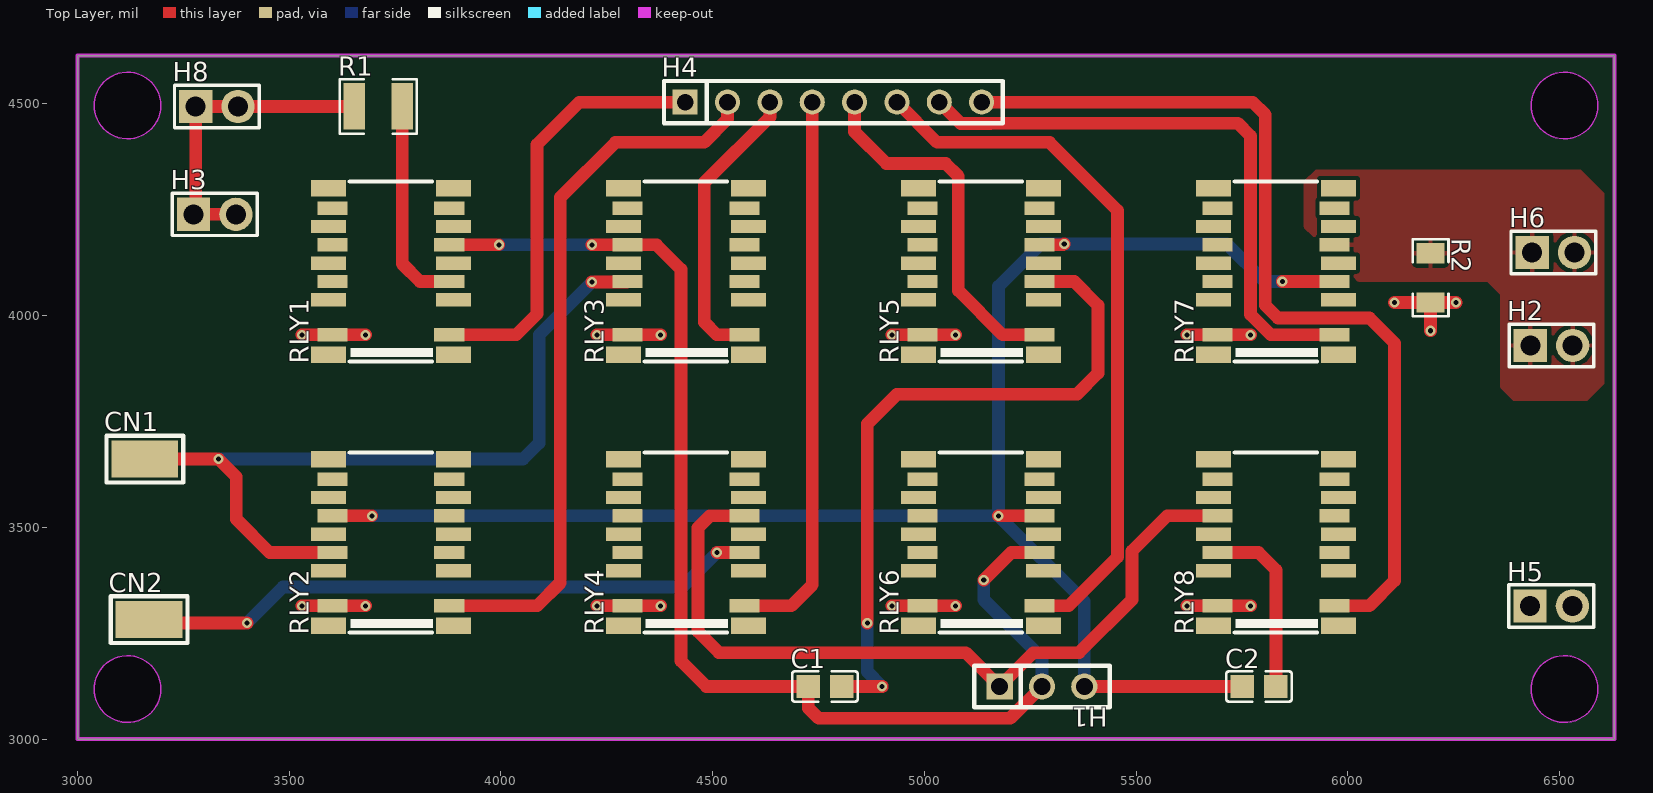
[diagram p0: Top Layer view]
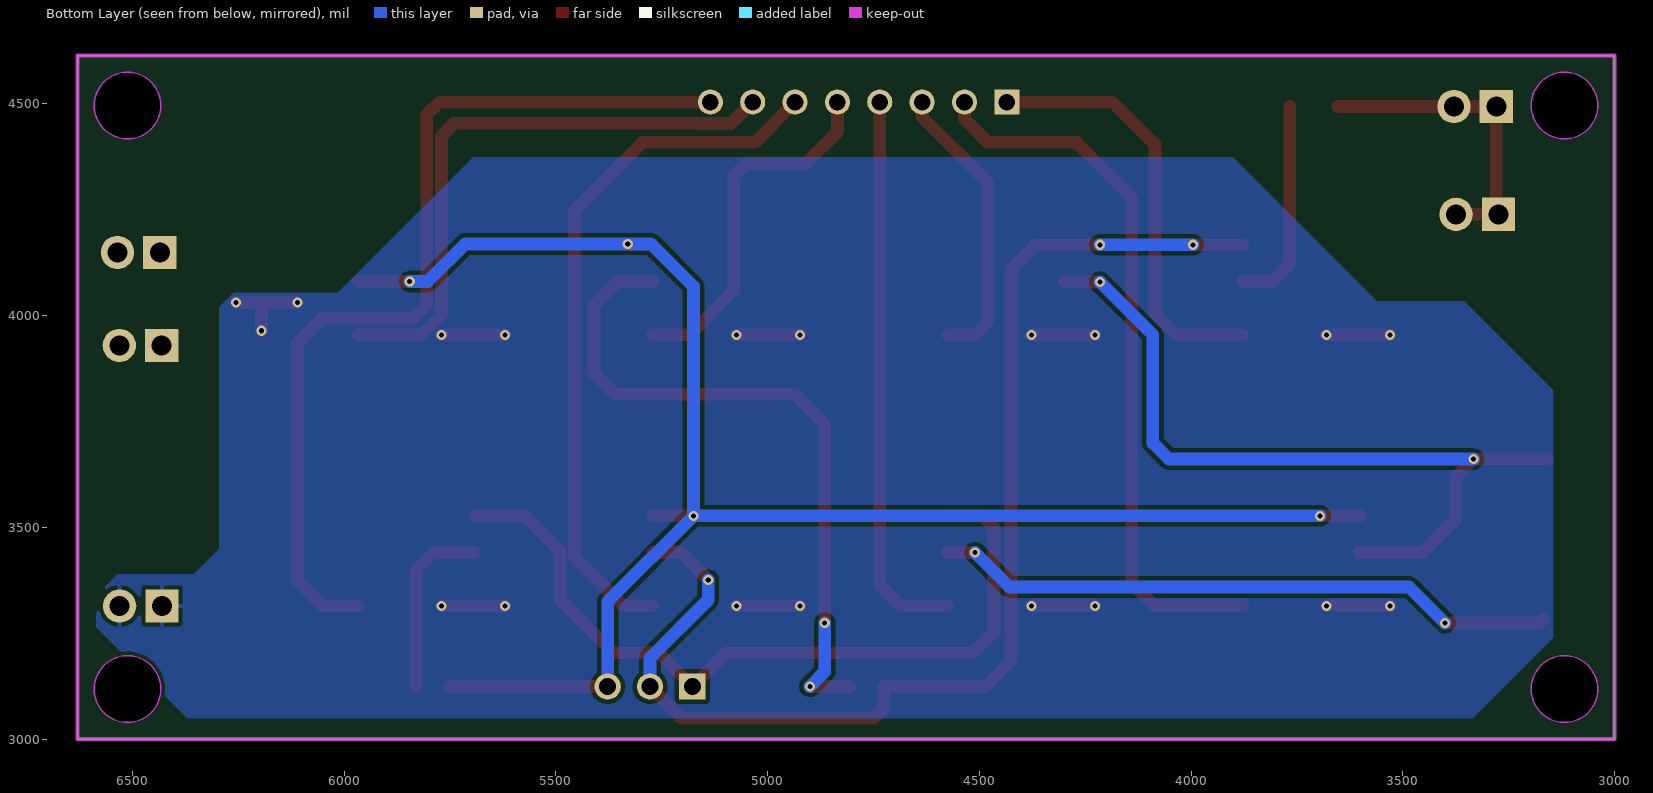
[diagram p1: Bottom Layer view, seen from below]
# Altium PCB MISC51843.pcbdoc
Units mil, origin at the board's own origin, x right, y up, seen from the top; angles counter-clockwise.
Board outline 3629.38 x 1614.17 mil, 2 copper layers (Top Layer, Bottom Layer), stack 62.206 mil thick; 21 components, 19 nets, 175 pads, 32 vias.

## Layer stack, top to bottom
Top Solder Mask Layer: solder mask 0.394, Dk 3.3
Top Layer: signal copper 1.379
Dielectric1: surface 59.449, FR4, Dk 4.5
Bottom Layer: signal copper 1.378
Bottom Solder Mask Layer: solder mask 0.394, Dk 3.3

## Board outline
3000,4614.17 3000,3000 6629.38,3000 6629.38,4614.17
cut-out: 3196.85,4496.06 cw(c3118.11,4496.06) 3039.37,4496.06 cw(c3118.11,4496.06)
cut-out: 6590.01,4496.06 cw(c6511.27,4496.06) 6432.53,4496.06 cw(c6511.27,4496.06)
cut-out: 6590.01,3118.11 cw(c6511.27,3118.11) 6432.53,3118.11 cw(c6511.27,3118.11)
cut-out: 3196.85,3118.11 cw(c3118.11,3118.11) 3039.37,3118.11 cw(c3118.11,3118.11)

## Design rules (kind name [scope] priority, off if disabled: settings)
BoardOutlineClearance copperThickness2oz_1 [All] p2 off: genericclearance=7.99 ignorepadtopadclearanceinfootprint=FALSE except(0: Arc-SplitContinuation Track-SplitContinuation SMDPad-SplitContinuation THPad-SplitContinuation Via-SplitContinuation Fill-SplitContinuation Region-SplitContinuation Poly-SplitContinuation Text-SplitContinuation Hole-SplitContinuation; 5.98: Arc-CutoutEdge SMDPad-CutoutEdge THPad-CutoutEdge Via-CutoutEdge Fill-CutoutEdge Region-CutoutEdge Text-CutoutEdge; 6.93: Hole-OutlineEdge Hole-CutoutEdge; 10: Poly-OutlineEdge Poly-CutoutEdge; 11.81: Arc-OutlineEdge Track-OutlineEdge SMDPad-OutlineEdge THPad-OutlineEdge Via-OutlineEdge Fill-OutlineEdge Region-OutlineEdge Text-OutlineEdge Track-CutoutEdge)
BoardOutlineClearance copperThickness1oz_1 [All] p4: genericclearance=4.02 ignorepadtopadclearanceinfootprint=FALSE except(0: Arc-SplitContinuation Track-SplitContinuation SMDPad-SplitContinuation THPad-SplitContinuation Via-SplitContinuation Fill-SplitContinuation Region-SplitContinuation Poly-SplitContinuation Text-SplitContinuation Hole-SplitContinuation; 6: SMDPad-CutoutEdge THPad-CutoutEdge Via-CutoutEdge Fill-CutoutEdge Region-CutoutEdge Text-CutoutEdge; 6.93: Hole-OutlineEdge Hole-CutoutEdge; 10: Poly-OutlineEdge Poly-CutoutEdge; 11.8: Arc-OutlineEdge Track-OutlineEdge SMDPad-OutlineEdge THPad-OutlineEdge Via-OutlineEdge Fill-OutlineEdge Region-OutlineEdge Text-OutlineEdge; 11.81: Arc-CutoutEdge Track-CutoutEdge)
Clearance copperThickness2oz [All] p1 off: gap=7.99 ignorepadtopadclearanceinfootprint=FALSE except(5.98: SMDPad-Track SMDPad-SMDPad THPad-Track SMDPad-THPad THPad-THPad Track-Via SMDPad-Via THPad-Via Via-Via Fill-Track Region-Track Fill-SMDPad Region-SMDPad Fill-THPad Region-THPad Fill-Via Region-Via Fill-Fill Fill-Region Region-Region Arc-Track Arc-SMDPad Arc-THPad Arc-Via Fill-Arc Region-Arc Arc-Arc Text-Track SMDPad-Text Text-THPad Text-Via Fill-Text Region-Text Arc-Text Text-Text; 6.93: Hole-Track Hole-SMDPad Hole-THPad Hole-Via Fill-Hole Region-Hole Hole-Arc Hole-Text; 10: Poly-Track Poly-SMDPad Poly-THPad Poly-Via Poly-Fill Poly-Region Poly-Poly Poly-Arc Poly-Text Poly-Hole)
Clearance copperThickness1oz [All] p3: gap=4.02 ignorepadtopadclearanceinfootprint=FALSE except(5.98: SMDPad-Track SMDPad-SMDPad THPad-Track SMDPad-THPad THPad-THPad Track-Via SMDPad-Via THPad-Via Via-Via Fill-Track Region-Track Fill-SMDPad Region-SMDPad Fill-THPad Region-THPad Fill-Via Region-Via Fill-Fill Fill-Region Region-Region; 6: Arc-Track Arc-SMDPad Arc-THPad Arc-Via Fill-Arc Region-Arc Arc-Arc Text-Track SMDPad-Text Text-THPad Text-Via Fill-Text Region-Text Arc-Text Text-Text; 6.93: Hole-Track Hole-SMDPad Hole-THPad Hole-Via Fill-Hole Region-Hole Hole-Arc Hole-Text; 10: Poly-Track Poly-SMDPad Poly-THPad Poly-Via Poly-Fill Poly-Region Poly-Poly Poly-Arc Poly-Text Poly-Hole)
Creepage creepage [All] p1: checkdistance=0 ignoreinternallayers=TRUE applytopolygonpour=TRUE
DiffPairsRouting differentialPair [All] p1: maxlimit=6 minlimit=6 mostfreqgap=6 toplayer_minwidth=5 toplayer_prefwidth=10 toplayer_maxwidth=100 toplayer_mingap=6 toplayer_prefgap=6 toplayer_maxgap=6 bottomlayer_minwidth=5 bottomlayer_prefwidth=10 bottomlayer_maxwidth=100 bottomlayer_mingap=6 bottomlayer_prefgap=6 bottomlayer_maxgap=6 maxuncoupledlength=10
HoleToHoleClearance otherClearance [All] p1: gap=11.81 allowstackedmicrovias=TRUE
Length netLength [All] p1: minlimit=0 maxlimit=0
MatchedLengths netLengthTolerance [All] p1: tolerance=1000
PasteMaskExpansion pasteMaskExpansion [All] p1: expansion=0
PlaneConnect innerPlane [All] p1: planeconnectstyle=Relief reliefexpansion=20 reliefentries=4 reliefconductorwidth=10 reliefairgap=10
PolygonConnect copperRegion [(InNet('$2N20') OR InNet('AGND'))] p1: connectstyle=Relief reliefconductorwidth=10 reliefentries=4 polygonreliefangle="90 Angle" airgapwidth=10 via.connectstyle=Relief via.reliefconductorwidth=10 via.reliefentries=4 via.polygonreliefangle="90 Angle" via.airgapwidth=10
RoutingVias viaSize [All] p1: holewidth=12.01 width=24.02 viastyle="Through Hole" minholewidth=11.81 minwidth=19.68 maxholewidth=248.03 maxwidth=393.7
SolderMaskExpansion solderMaskExpansion [IsVia] p1: expansion=-1000 istentingtop=TRUE
SolderMaskExpansion solderMaskExpansion [All] p2: expansion=2 istentingtop=FALSE
Width copperThickness2oz_2 [All] p1 off: maxlimit=100 minlimit=8 preferedwidth=10
Width copperThickness1oz_2 [All] p2: maxlimit=100 minlimit=5 preferedwidth=10

## Components (designator, comment, footprint, x,y, rotation, side; value= is the part's Value field where it differs from the comment)
C1 "470nF" C0805 4765,3124.17 r0 top
C2 "470nF" C0805 5790,3124.17 r0 top
CN1 "RH-5019" TESTPOINT-SMD_L3.8-W2.0_RH-5019 3159,3661.23 r0 top
CN2 "RH-5019" TESTPOINT-SMD_L3.8-W2.0_RH-5019 3169,3282.2 r0 top
H1 "PM254V-11-03-H85" HDR-TH_3P-P2.54-V-F 5277.5,3124.17 r0 top
H2 "PZ254V-11-02P" HDR-TH_2P-P2.54-V-M 6480.67,3929.55 r0 top
H3 "PZ254V-11-02P" HDR-TH_2P-P2.54-V-M 3324,4239.17 r0 top
H4 "PZ254V-11-08P" HDR-TH_8P-P2.54-V-M 4785,4504.17 r0 top
H5 "PZ254V-11-02P" HDR-TH_2P-P2.54-V-M 6480,3314.17 r0 top
H6 "PZ254V-11-02P" HDR-TH_2P-P2.54-V-M 6485,4149.17 r0 top
H8 "PZ254V-11-02P" HDR-TH_2P-P2.54-V-M 3329,4493.86 r0 top
R1 "1kΩ" R1210 3710,4494.17 r0 top
R2 "0Ω" R1206 6195,4089.17 r270 top
RLY1 "G6K-2F-RF-S DC5" RELAY-SMD_G6K-2F-RF-S-DC12 3740,4104.17 r90 top
RLY2 "G6K-2F-RF-S DC5" RELAY-SMD_G6K-2F-RF-S-DC12 3740,3464.17 r90 top
RLY3 "G6K-2F-RF-S DC5" RELAY-SMD_G6K-2F-RF-S-DC12 4436.67,4104.17 r90 top
RLY4 "G6K-2F-RF-S DC5" RELAY-SMD_G6K-2F-RF-S-DC12 4436.67,3464.17 r90 top
RLY5 "G6K-2F-RF-S DC5" RELAY-SMD_G6K-2F-RF-S-DC12 5133.33,4104.17 r90 top
RLY6 "G6K-2F-RF-S DC5" RELAY-SMD_G6K-2F-RF-S-DC12 5133.33,3464.17 r90 top
RLY7 "G6K-2F-RF-S DC5" RELAY-SMD_G6K-2F-RF-S-DC12 5830,4104.17 r90 top
RLY8 "G6K-2F-RF-S DC5" RELAY-SMD_G6K-2F-RF-S-DC12 5830,3464.17 r90 top

## Footprints (in the part's own frame and the unit in brackets; to place one, negate y for a bottom-side part, rotate by r counter-clockwise, add the part's x,y. Pads: shape width x height; smd on the part's side, far side on the other; paste and mask are expansions set on the pad)
C0805 [mm]
  rect 1.41x1.35 smd paste-100 mask+0.051: 1(-1,0) 2(1,0)
  silkscreen extent -1.96,-0.9 1.96,0.9
HDR-TH_2P-P2.54-V-M [mm]
  rect 2x2 hole 1.2: 1(-1.27,0)
  round 2 hole 1.2: 2(1.27,0)
  silkscreen extent -2.54,-1.27 2.54,1.27
HDR-TH_3P-P2.54-V-F [mil]
  rect 62x62 hole 40.16: 1(-100,0)
  round 62 hole 40.16: 2(0,0) 3(100,0)
  silkscreen extent -160,-49 160,49
HDR-TH_8P-P2.54-V-M [mm]
  rect 1.5x1.5 hole 1: 1(-8.89,0)
  round 1.5 hole 1: 2(-6.35,0) 3(-3.81,0) 4(-1.27,0) 5(1.27,0) 6(3.81,0) 7(6.35,0) 8(8.89,0)
  silkscreen extent -10.16,-1.27 10.16,1.27
R1206 [mil]
  rect 47.54x66.97 smd paste-3937.01 mask+2: 1(-58.22,0) 2(58.22,0)
  silkscreen extent -91,-42 91,42
R1210 [mil]
  rect 50.49x110.55 smd paste-3937.01 mask+2: 1(-56.74,0) 2(56.74,0)
  silkscreen extent -91,-64 91,64
RELAY-SMD_G6K-2F-RF-S-DC12 [mm]
  rect 0.8x1.8 smd: 1(-3.8,-3.5) 2(-0.6,-3.5) 3(1.6,-3.5) 4(3.8,-3.5) 5(3.8,3.5) 6(1.6,3.5) 7(-0.6,3.5) 8(-3.8,3.5)
  rect 1x2.1 smd: 9(-5,3.75) 10(-5,-3.75) 14(5,-3.75) 15(5,3.75)
  rect 0.8x2.1 smd: 11(-1.7,-3.75) 12(0.5,-3.75) 13(2.7,-3.75) 16(2.7,3.75) 17(0.5,3.75) 18(-1.7,3.75)
  silkscreen extent -5.4,-2.5 5.4,2.47
TESTPOINT-SMD_L3.8-W2.0_RH-5019 [mm]
  rect 4x2.2 smd: 1(0,0)
  silkscreen extent -2.3,-1.4 2.3,1.4

## Via types
v1: diameter 24.02, hole 12, Top Layer to Bottom Layer, 32 vias

## Nets (pads, with @x,y where several pads share a name; then routed paths per layer and width w, separated by ;. In a path a pad name is that pad's centre, name@x,y a point inside that pad or via, vN(x,y) a via of type N, cw(c..) or ccw(c..) an arc to the next point about the centre after c; other vN are vias at no path point)
$2N18: R1.2 RLY1.2 | length 500.1
  Top Layer w30: R1.2 3766.74,4122.43 3808.63,4080.54 RLY1.2
$2N19: C1.1 H1.2 RLY1.3 RLY3.6 RLY6.2 | length 2931.7
  Top Layer w30: RLY1.3 v1(3995,4167.16) ; v1(4215,4167.16) RLY3.6 4367.01,4167.16 4425,4109.17 4425,3184.17 4485,3124.17 C1.1 4725.63,3073.54 4750,3049.17 5202.5,3049.17 H1.2 ; v1(5140,3375.54) 5205,3440.54 RLY6.2
  Bottom Layer w30: v1(3995,4167.16) v1(4215,4167.16) ; v1(5140,3375.54) 5140,3329.17 5277.5,3191.67 H1.2
$2N20: C2.1 H1.3 RLY2.6 RLY5.3 RLY6.3 RLY7.2 | length 4001.6
  Top Layer w30: RLY2.6 v1(3695,3527.16) ; v1(5175,3527.16) RLY6.3 ; RLY5.3 5327.99,4167.16 v1(5330,4169.17) ; H1.3 C2.1 ; v1(5845,4080.54) RLY7.2
  Bottom Layer w30: v1(3695,3527.16) v1(5175,3527.16) ; H1.3 5377.5,3324.66 v1(5175,3527.16) ; v1(5845,4080.54) 5802.57,4080.54 5713.94,4169.17 v1(5330,4169.17) 5275,4169.17 5175,4069.17 v1(5175,3527.16)
$2N24: H1.1 RLY4.3 RLY8.6 | length 1881.4
  Top Layer w30: RLY4.3 4492.99,3527.16 4465,3499.17 4465,3254.17 4515,3204.17 5097.5,3204.17 H1.1 5257.5,3204.17 5365,3204.17 5490,3329.17 5490,3444.17 5572.99,3527.16 RLY8.6
$2N28: C1.2 RLY5.2 | length 1647.1
  Top Layer w30: C1.2 v1(4900,3124.17) ; v1(4865,3274.17) 4865,3744.17 4935,3814.17 5360,3814.17 5410,3864.17 5410,4024.17 5353.63,4080.54 RLY5.2
  Bottom Layer w30: v1(4865,3274.17) 4865,3159.17 v1(4900,3124.17)
$2N37: C2.2 RLY8.7 | length 430.2
  Top Layer w30: RLY8.7 5788.63,3440.54 5830,3399.17 5830,3124.8 C2.2
AGND: H2.1 H2.2 H6.1 H6.2 R2.1 RLY7.3
CTRL1: H4.1 RLY1.1 | length 1019.2
  Top Layer w30: RLY1.1 4035.39,3954.56 4085,4004.17 4085,4404.17 4185,4504.17 H4.1
CTRL2: H4.2 RLY2.1 | length 1706.5
  Top Layer w30: RLY2.1 4085.39,3314.56 4140,3369.17 4140,4279.17 4270,4409.17 4480,4409.17 4535,4464.17 H4.2
CTRL3: H4.3 RLY3.1 | length 690.7
  Top Layer w30: RLY3.1 4510,3954.56 4480,3984.56 4480,4314.17 4635,4469.17 H4.3
CTRL4: H4.4 RLY4.1 | length 1321.1
  Top Layer w30: RLY4.1 4685.39,3314.56 4735,3364.17 H4.4
CTRL5: H4.5 RLY5.1 | length 863
  Top Layer w30: H4.5 4835,4434.17 4910,4359.17 5050,4359.17 5080,4329.17 5080,4059.17 5184.61,3954.56 RLY5.1
CTRL6: H4.6 RLY6.1 | length 1677.8
  Top Layer w30: H4.6 5030,4409.17 5295,4409.17 5455.98,4248.19 5455.98,3430.16 5340.39,3314.56 RLY6.1
CTRL7: H4.7 RLY7.1 | length 1407.8
  Top Layer w30: H4.7 5085.51,4453.66 5155.92,4453.66 5156.43,4454.17 5740,4454.17 5770,4424.17 5770,4002.67 5818.11,3954.56 RLY7.1
CTRL8: H4.8 RLY8.1 | length 2202.1
  Top Layer w30: H4.8 5775,4504.17 5805,4474.17 5805,4024.17 5835,3994.17 6050.91,3994.17 6110,3935.08 6110,3374.17 6050.39,3314.56 RLY8.1
DGND: H5.1 H5.2 R2.2 RLY1.8 RLY2.8 RLY3.8 RLY4.8 RLY5.8 RLY6.8 RLY7.8 RLY8.8 | length 1411.8
  Top Layer w30: v1(3530,3314.56) RLY2.8 v1(3680,3314.56) ; v1(3530,3954.56) RLY1.8 v1(3680,3954.56) ; v1(4226.67,3314.56) RLY4.8 v1(4376.67,3314.56) ; v1(4226.67,3954.56) RLY3.8 v1(4376.67,3954.56) ; v1(4923.33,3314.56) RLY6.8 v1(5073.33,3314.56) ; v1(4923.33,3954.56) RLY5.8 v1(5073.33,3954.56) ; v1(5620,3314.56) RLY8.8 v1(5770,3314.56) ; v1(5620,3954.56) RLY7.8 v1(5770,3954.56) ; v1(6110,4030.95) R2.2 ; v1(6195,3964.17) R2.2 ; v1(6255,4030.95) R2.2
HH: CN2.1 RLY4.2 | length 1477.7
  Top Layer w30: CN2.1 3177.03,3274.17 v1(3400,3274.17) ; v1(4510,3440.54) RLY4.2
  Bottom Layer w30: v1(3400,3274.17) 3485,3359.17 4428.63,3359.17 v1(4510,3440.54)
LL: CN1.1 RLY2.7 RLY3.7 | length 1882.2
  Top Layer w30: CN1.1 v1(3332.94,3661.23) 3375,3619.17 3375,3519.17 3453.63,3440.54 RLY2.7 ; v1(4215,4079.17) 4297.5,4079.17 RLY3.7
  Bottom Layer w30: v1(3332.94,3661.23) 4052.06,3661.23 4090,3699.17 4090,3954.17 v1(4215,4079.17)
VDD: H3.1 H3.2 H8.1 H8.2 R1.1 | length 731.1
  Top Layer w30: H3.2 H3.1 3279,4244.17 H8.1 H8.2 3652.95,4493.86 R1.1
pads on no net: RLY1.4 RLY1.5 RLY1.6 RLY1.7 RLY1.9 RLY1.10 RLY1.11 RLY1.12 RLY1.13 RLY1.14 RLY1.15 RLY1.16 RLY1.17 RLY1.18 RLY2.2 RLY2.3 RLY2.4 RLY2.5 RLY2.9 RLY2.10 RLY2.11 RLY2.12 RLY2.13 RLY2.14 RLY2.15 RLY2.16 RLY2.17 RLY2.18 RLY3.2 RLY3.3 RLY3.4 RLY3.5 RLY3.9 RLY3.10 RLY3.11 RLY3.12 RLY3.13 RLY3.14 RLY3.15 RLY3.16 RLY3.17 RLY3.18 RLY4.4 RLY4.5 RLY4.6 RLY4.7 RLY4.9 RLY4.10 RLY4.11 RLY4.12 RLY4.13 RLY4.14 RLY4.15 RLY4.16 RLY4.17 RLY4.18 RLY5.4 RLY5.5 RLY5.6 RLY5.7 RLY5.9 RLY5.10 RLY5.11 RLY5.12 RLY5.13 RLY5.14 RLY5.15 RLY5.16 RLY5.17 RLY5.18 RLY6.4 RLY6.5 RLY6.6 RLY6.7 RLY6.9 RLY6.10 RLY6.11 RLY6.12 RLY6.13 RLY6.14 RLY6.15 RLY6.16 RLY6.17 RLY6.18 RLY7.4 RLY7.5 RLY7.6 RLY7.7 RLY7.9 RLY7.10 RLY7.11 RLY7.12 RLY7.13 RLY7.14 RLY7.15 RLY7.16 RLY7.17 RLY7.18 RLY8.2 RLY8.3 RLY8.4 RLY8.5 RLY8.9 RLY8.10 RLY8.11 RLY8.12 RLY8.13 RLY8.14 RLY8.15 RLY8.16 RLY8.17 RLY8.18

## Polygon pours and split planes (outlines as drawn)
DGND on Bottom Layer (solid, remove dead copper, pour order 2): 3561.12,4034.17 3901.12,4374.17 5695,4374.17 6015,4054.17 6260,4054.17 6295,4019.17 6295,3449.17 6355,3389.17 6535,3389.17 6585,3339.17 6585,3264.17 6370,3049.17 3335,3049.17 3145,3239.17 3145,3824.17 3355,4034.17
AGND on Top Layer (solid, remove dead copper, pour order 0): 5896.15,4316.77 5923.56,4344.17 6550,4344.17 6605,4289.17 6605,3839.17 6565,3799.17 6390,3799.17 6360,3829.17 6360,4049.17 6328.63,4080.54 6023.63,4080.54 5896.15,4208.02

## Keep-outs
Board Outline Layer:
  region: 3196.85,4496.06 cw(c3118.11,4496.06) 3039.37,4496.06 cw(c3118.11,4496.06)
  circle w0.1: c3118.11,4496.06 r78.74
  region: 3196.85,4496.06 3196.47,4488.35 3195.34,4480.7 3193.46,4473.21 3190.86,4465.93 3187.55,4458.95 3183.58,4452.32 3178.98,4446.11 3173.79,4440.39 3168.06,4435.2 3161.86,4430.59 3155.23,4426.62 3148.24,4423.32 3140.97,4420.71 3133.47,4418.84 3125.83,4417.7 3118.11,4417.32 3110.39,4417.7 3102.75,4418.84 3095.25,4420.71 3087.98,4423.32 3080.99,4426.62 3074.36,4430.59 3068.16,4435.2 3062.43,4440.39 3057.24,4446.11 3052.64,4452.32 3048.67,4458.95 3045.36,4465.93 3042.76,4473.21 3040.88,4480.7 3039.75,4488.35 3039.37,4496.06 3039.75,4503.78 3040.88,4511.42 3042.76,4518.92 3045.36,4526.2 3048.67,4533.18 3052.64,4539.81 3057.24,4546.02 3062.43,4551.74 3068.16,4556.93 3074.36,4561.53 3080.99,4565.51 3087.98,4568.81 3095.25,4571.41 3102.75,4573.29 3110.39,4574.42 3118.11,4574.8 3125.83,4574.42 3133.47,4573.29 3140.97,4571.41 3148.24,4568.81 3155.23,4565.51 3161.86,4561.53 3168.06,4556.93 3173.79,4551.74 3178.98,4546.02 3183.58,4539.81 3187.55,4533.18 3190.86,4526.2 3193.46,4518.92 3195.34,4511.42 3196.47,4503.78
  region: 6590.01,4496.06 cw(c6511.27,4496.06) 6432.53,4496.06 cw(c6511.27,4496.06)
  circle w0.1: c6511.27,4496.06 r78.74
  region: 6590.01,4496.06 6589.63,4488.35 6588.5,4480.7 6586.62,4473.21 6584.02,4465.93 6580.72,4458.95 6576.74,4452.32 6572.14,4446.11 6566.95,4440.39 6561.23,4435.2 6555.02,4430.59 6548.39,4426.62 6541.41,4423.32 6534.13,4420.71 6526.63,4418.84 6518.99,4417.7 6511.27,4417.32 6503.56,4417.7 6495.91,4418.84 6488.42,4420.71 6481.14,4423.32 6474.16,4426.62 6467.53,4430.59 6461.32,4435.2 6455.6,4440.39 6450.41,4446.11 6445.8,4452.32 6441.83,4458.95 6438.53,4465.93 6435.92,4473.21 6434.05,4480.7 6432.91,4488.35 6432.53,4496.06 6432.91,4503.78 6434.05,4511.42 6435.92,4518.92 6438.53,4526.2 6441.83,4533.18 6445.8,4539.81 6450.41,4546.02 6455.6,4551.74 6461.32,4556.93 6467.53,4561.53 6474.16,4565.51 6481.14,4568.81 6488.42,4571.41 6495.91,4573.29 6503.56,4574.42 6511.27,4574.8 6518.99,4574.42 6526.63,4573.29 6534.13,4571.41 6541.41,4568.81 6548.39,4565.51 6555.02,4561.53 6561.23,4556.93 6566.95,4551.74 6572.14,4546.02 6576.74,4539.81 6580.72,4533.18 6584.02,4526.2 6586.62,4518.92 6588.5,4511.42 6589.63,4503.78
  region: 6590.01,3118.11 cw(c6511.27,3118.11) 6432.53,3118.11 cw(c6511.27,3118.11)
  circle w0.1: c6511.27,3118.11 r78.74
  region: 6590.01,3118.11 6589.63,3110.39 6588.5,3102.75 6586.62,3095.25 6584.02,3087.98 6580.72,3080.99 6576.74,3074.36 6572.14,3068.16 6566.95,3062.43 6561.23,3057.24 6555.02,3052.64 6548.39,3048.67 6541.41,3045.36 6534.13,3042.76 6526.63,3040.88 6518.99,3039.75 6511.27,3039.37 6503.56,3039.75 6495.91,3040.88 6488.42,3042.76 6481.14,3045.36 6474.16,3048.67 6467.53,3052.64 6461.32,3057.24 6455.6,3062.43 6450.41,3068.16 6445.8,3074.36 6441.83,3080.99 6438.53,3087.98 6435.92,3095.25 6434.05,3102.75 6432.91,3110.39 6432.53,3118.11 6432.91,3125.83 6434.05,3133.47 6435.92,3140.97 6438.53,3148.24 6441.83,3155.23 6445.8,3161.86 6450.41,3168.06 6455.6,3173.79 6461.32,3178.98 6467.53,3183.58 6474.16,3187.55 6481.14,3190.86 6488.42,3193.46 6495.91,3195.34 6503.56,3196.47 6511.27,3196.85 6518.99,3196.47 6526.63,3195.34 6534.13,3193.46 6541.41,3190.86 6548.39,3187.55 6555.02,3183.58 6561.23,3178.98 6566.95,3173.79 6572.14,3168.06 6576.74,3161.86 6580.72,3155.23 6584.02,3148.24 6586.62,3140.97 6588.5,3133.47 6589.63,3125.83
  region: 3196.85,3118.11 cw(c3118.11,3118.11) 3039.37,3118.11 cw(c3118.11,3118.11)
  circle w0.1: c3118.11,3118.11 r78.74
  region: 3196.85,3118.11 3196.47,3110.39 3195.34,3102.75 3193.46,3095.25 3190.86,3087.98 3187.55,3080.99 3183.58,3074.36 3178.98,3068.16 3173.79,3062.43 3168.06,3057.24 3161.86,3052.64 3155.23,3048.67 3148.24,3045.36 3140.97,3042.76 3133.47,3040.88 3125.83,3039.75 3118.11,3039.37 3110.39,3039.75 3102.75,3040.88 3095.25,3042.76 3087.98,3045.36 3080.99,3048.67 3074.36,3052.64 3068.16,3057.24 3062.43,3062.43 3057.24,3068.16 3052.64,3074.36 3048.67,3080.99 3045.36,3087.98 3042.76,3095.25 3040.88,3102.75 3039.75,3110.39 3039.37,3118.11 3039.75,3125.83 3040.88,3133.47 3042.76,3140.97 3045.36,3148.24 3048.67,3155.23 3052.64,3161.86 3057.24,3168.06 3062.43,3173.79 3068.16,3178.98 3074.36,3183.58 3080.99,3187.55 3087.98,3190.86 3095.25,3193.46 3102.75,3195.34 3110.39,3196.47 3118.11,3196.85 3125.83,3196.47 3133.47,3195.34 3140.97,3193.46 3148.24,3190.86 3155.23,3187.55 3161.86,3183.58 3168.06,3178.98 3173.79,3173.79 3178.98,3168.06 3183.58,3161.86 3187.55,3155.23 3190.86,3148.24 3193.46,3140.97 3195.34,3133.47 3196.47,3125.83
  lines w10: 3000,3000 3000,4614.17 6629.38,4614.17 6629.38,3000 3000,3000

## Silkscreen, mask and mechanical layers (free items; w line width, h text height)
Mechanical Layer:
  circle w0.1: c3118.11,4496.06 r78.74
  circle w0.1: c6511.27,4496.06 r78.74
  circle w0.1: c6511.27,3118.11 r78.74
  circle w0.1: c3118.11,3118.11 r78.74

## Dimensions
3000,4657.68 to 6629.38,4657.68 on Document Layer
6810,4614.17 to 6810,3000 on Document Layer